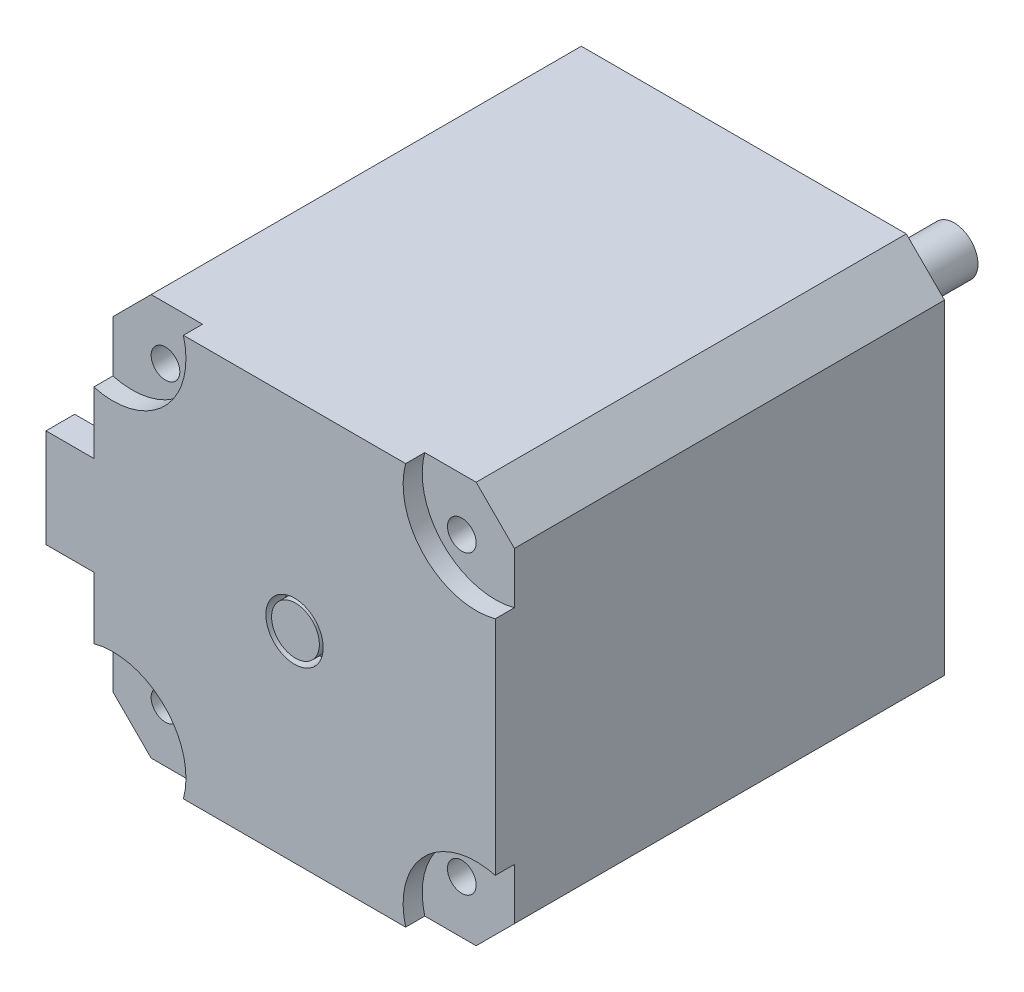
SolidWorks part; units mm, degrees
ref_plane "Front Plane" through (0, 0, 0) normal (0, 0, 1) x (1, 0, 0)
ref_plane "Top Plane" through (0, 0, 0) normal (0, 1, 0) x (1, 0, 0)
ref_plane "Right Plane" through (0, 0, 0) normal (1, 0, 0) x (0, 0, -1)
sketch "Sketch1" plane through (0, 0, 0) normal (0, 0, 1) x (1, 0, 0)
  line L0 (0, 21) -> (0, -21) construction
  line L1 (-21, 21) -> (21, 21)
  line L2 (-21, 21) -> (-21, -21)
  line L3 (-21, -21) -> (21, -21)
  line L4 (21, 21) -> (21, -21)
  line L5 (-21, 21) -> (21, -21) construction
  line L6 (-21, -21) -> (21, 21) construction
  line L7 (-21, 0) -> (21, 0) construction
  circle A0 centre (-15.5, 15.5) radius 1.5
  circle A1 centre (15.5, 15.5) radius 1.5
  circle A2 centre (-15.5, -15.5) radius 1.5
  circle A3 centre (15.5, -15.5) radius 1.5
  point P0 (0, 0)
  dimension "D2" = 31
  dimension "D3" = 3
  dimension "D1" = 42
  dimension "D4" = 42
extrude "Boss-Extrude1" add sketch "Sketch1" along normal blind 47
sketch "Sketch3" plane through (0, 0, 0) normal (0, 0, -1) x (-1, 0, 0)
  line L0 (-21, 17) -> (-17, 21)
  line L1 (-21, -21) -> (-21, 21) construction
  line L2 (-21, 21) -> (21, 21) construction
  line L3 (0, 18.9412) -> (0, -7.5636) construction
  line L4 (-16.264, 0) -> (-4.6279, 0) construction
  line L5 (-21, 21) -> (-21, 17)
  line L6 (-21, 21) -> (-17, 21)
  line L7 (21, 21) -> (17, 21)
  line L8 (21, 21) -> (21, 17)
  line L9 (21, 17) -> (17, 21)
  line L10 (21, -17) -> (17, -21)
  line L11 (21, -21) -> (21, -17)
  line L12 (21, -21) -> (17, -21)
  line L13 (-21, -21) -> (-17, -21)
  line L14 (-21, -21) -> (-21, -17)
  line L15 (-21, -17) -> (-17, -21)
  dimension "D1" = 4
  dimension "D2" = 4
extrude "Cut-Extrude1" cut sketch "Sketch3" against normal through all
sketch "Sketch4" plane through (0, 0, 0) normal (0, 0, -1) x (-1, 0, 0)
  circle A0 centre (0, 0) radius 11
  dimension "D1" = 22
extrude "Boss-Extrude2" add sketch "Sketch4" along normal blind 2
sketch "Sketch5" plane through (0, 0, -2) normal (0, 0, -1) x (-1, 0, 0)
  line L0 (1.7, -1.833) -> (1.7, 1.833)
  arc A0 (1.7, 1.833) -> (1.7, -1.833) centre (0, 0) ccw
  dimension "D1" = 5
  dimension "D2" = 1.7
extrude "Boss-Extrude3" add sketch "Sketch5" along normal blind 20
sketch "Sketch7" plane through (0, 0, 47) normal (0, 0, 1) x (1, 0, 0)
  line L0 (-17, 21) -> (-21, 17) construction
  line L9 (0, 13.3214) -> (0, 5.5116) construction
  line L10 (-12.44, 0) -> (-6.0632, 0) construction
  line L11 (21, 17) -> (21, 11.6255)
  line L12 (17, 21) -> (21, 17)
  line L13 (11.6255, 21) -> (17, 21)
  line L14 (-21, -17) -> (-21, -11.6255)
  line L15 (-17, -21) -> (-21, -17)
  line L16 (-11.6255, -21) -> (-17, -21)
  line L17 (17, -21) -> (21, -17)
  line L18 (21, -17) -> (21, 17)
  line L19 (21, 17) -> (17, 21)
  line L20 (17, 21) -> (-17, 21)
  line L21 (-17, 21) -> (-21, 17)
  line L22 (-21, 17) -> (-21, -17)
  line L23 (-21, -17) -> (-17, -21)
  line L24 (-17, -21) -> (17, -21)
  line L28 (-11.6255, 21) -> (-17, 21)
  line L29 (-17, 21) -> (-21, 17)
  line L30 (-21, 17) -> (-21, 11.6255)
  line L33 (11.6255, -21) -> (17, -21)
  line L34 (17, -21) -> (21, -17)
  line L35 (21, -17) -> (21, -11.6255)
  arc A0 (-21, 11.6255) -> (-11.6255, 21) centre (-19, 19) ccw
  arc A1 (21, 11.6255) -> (11.6255, 21) centre (19, 19) cw
  arc A2 (21, -11.6255) -> (11.6255, -21) centre (19, -19) ccw
  arc A3 (-21, -11.6255) -> (-11.6255, -21) centre (-19, -19) cw
  dimension "D1" = 0
extrude "Cut-Extrude2" cut sketch "Sketch7" against normal blind 2
sketch "Sketch8" plane through (0, 0, 47) normal (0, 0, 1) x (1, 0, 0)
  circle A0 centre (0, 0) radius 3
  dimension "D1" = 6
extrude "Cut-Extrude3" cut sketch "Sketch8" against normal blind 2
sketch "Sketch9" plane through (0, 0, 45) normal (0, 0, 1) x (1, 0, 0)
  circle A0 centre (0, 0) radius 2.5
  dimension "D1" = 5
extrude "Boss-Extrude4" add sketch "Sketch9" along normal blind 1.9
sketch "Sketch10" plane through (-21, 0, 0) normal (-1, 0, 0) x (0, 0, 1)
  line L5 (47, 11.6255) -> (47, -11.6255) construction
  line L6 (44, 5.155) -> (47, 5.155)
  line L7 (44, 5.155) -> (44, -5.155)
  line L8 (44, -5.155) -> (47, -5.155)
  line L9 (47, 5.155) -> (47, -5.155)
  line L10 (44, 5.155) -> (47, -5.155) construction
  line L11 (44, -5.155) -> (47, 5.155) construction
  line L13 (44.2607, 4.2591) -> (46.7393, 4.2591)
  line L14 (44.2607, 4.2591) -> (44.2607, -4.2591)
  line L15 (44.2607, -4.2591) -> (46.7393, -4.2591)
  line L16 (46.7393, 4.2591) -> (46.7393, -4.2591)
  line L17 (44.2607, 4.2591) -> (46.7393, -4.2591) construction
  line L18 (44.2607, -4.2591) -> (46.7393, 4.2591) construction
  point P0 (45.5, 0)
  point P7 (45.5, 0)
  dimension "D1" = 3
extrude "Boss-Extrude5" add sketch "Sketch10" along normal blind 5
sketch "Sketch11" plane through (-21, 0, 0) normal (-1, 0, 0) x (0, 0, 1)
  line L0 (45.5, 4.2591) -> (45.5, -4.2591) construction
  line L1 (46.7393, 4.2591) -> (44.2607, 4.2591) construction
  line L2 (44.2607, -4.2591) -> (46.7393, -4.2591) construction
  circle A0 centre (45.5, 3.1278) radius 0.5
  circle A1 centre (45.5, 1.6278) radius 0.5
  circle A2 centre (45.5, 0.1278) radius 0.5
  circle A3 centre (45.5, -1.3722) radius 0.5
  circle A4 centre (45.5, -2.8722) radius 0.5
  dimension "D1" = 1
  dimension "D2" = 5
extrude "Boss-Extrude6" add sketch "Sketch11" along normal blind 5
